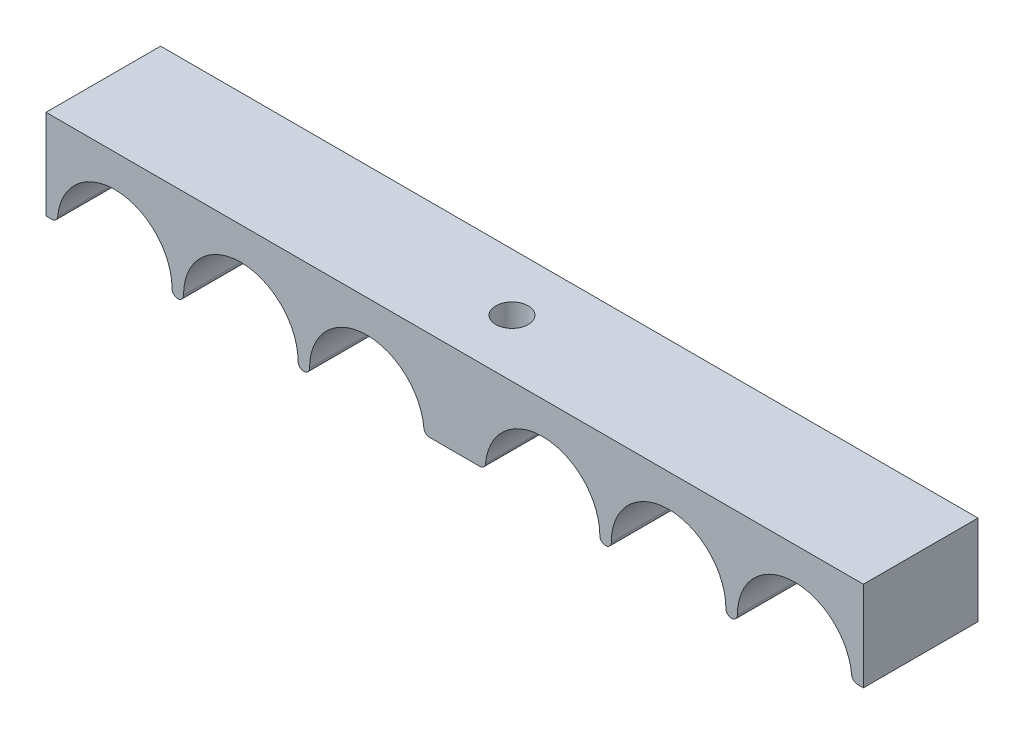
SolidWorks part; units mm, degrees
ref_plane "Front Plane" through (0, 0, 0) normal (0, 0, 1) x (1, 0, 0)
ref_plane "Top Plane" through (0, 0, 0) normal (0, 1, 0) x (1, 0, 0)
ref_plane "Right Plane" through (0, 0, 0) normal (1, 0, 0) x (0, 0, -1)
sketch "Sketch1" plane through (0, 0, 0) normal (0, 0, 1) x (1, 0, 0)
  line L0 (-107, 0) -> (-107, 23.5)
  line L1 (-107, 23.5) -> (107, 23.5)
  line L2 (107, 0) -> (-107, 0) construction
  line L3 (-89, 47.3416) -> (-89, -26.6733) construction
  line L4 (-107, 0) -> (-105.4317, 0)
  line L5 (-56, 0) -> (-56, -36.4967) construction
  line L6 (-23, 0) -> (-23, -38.0165) construction
  line L7 (6.5683, 0) -> (-6.5683, 0)
  line L8 (0, 0) -> (0, 56.3433) construction
  line L9 (107, 0) -> (105.4317, 0)
  line L10 (107, 0) -> (107, 23.5)
  arc A0 (-74, 0) -> (-103.9379, 1.3636) centre (-89, 0) ccw
  arc A1 (-41, 0) -> (-71, 0) centre (-56, 0) ccw
  arc A2 (-8.0621, 1.3636) -> (-38, 0) centre (-23, 0) ccw
  arc A3 (-105.4317, 0) -> (-103.9379, 1.3636) centre (-105.4317, 1.5) ccw
  arc A4 (-74, 0) -> (-71, 0) centre (-72.5, 0) ccw
  arc A5 (-41, 0) -> (-38, 0) centre (-39.5, 0) ccw
  arc A6 (-8.0621, 1.3636) -> (-6.5683, 0) centre (-6.5683, 1.5) ccw
  arc A7 (8.0621, 1.3636) -> (6.5683, 0) centre (6.5683, 1.5) cw
  arc A8 (41, 0) -> (38, 0) centre (39.5, 0) cw
  arc A9 (74, 0) -> (71, 0) centre (72.5, 0) cw
  arc A10 (105.4317, 0) -> (103.9379, 1.3636) centre (105.4317, 1.5) cw
  arc A11 (8.0621, 1.3636) -> (38, 0) centre (23, 0) cw
  arc A12 (41, 0) -> (71, 0) centre (56, 0) cw
  arc A13 (74, 0) -> (103.9379, 1.3636) centre (89, 0) cw
  point P42 (0, 23.5)
  dimension "D4" = 30
  dimension "D8" = 1.5
  dimension "D7" = 1.5
  dimension "D1" = 107
  dimension "D2" = 23.5
  dimension "D3" = 18
  dimension "D6" = 33
  dimension "D5" = 3
extrude "Boss-Extrude1" add sketch "Sketch1" along normal blind 30
hole_wizard "M10 Tapped Hole1" positions "Sketch3" profile "Sketch4" tap size "M10" standard "GB" end condition through all
sketch "Sketch3" plane through (0, 23.5, 0) normal (0, 1, 0) x (-1, 0, 0)
  line L0 (-107, 0) -> (107, 0) construction
  line L1 (107, 30) -> (107, 0) construction
  point P0 (0, 15)
  dimension "D1" = 15
  dimension "D2" = 107
sketch "Sketch4" plane through (0, 23.5, 15) normal (1, 0, 0) x (0, 0, 1)
  line L0 (0, 0) -> (0, 25)
  line L1 (0, 25) -> (4.25, 25)
  line L2 (4.25, 25) -> (4.25, 0)
  line L5 (4.25, 0) -> (0, 0)
  line L11 (0, -6.35) -> (0, 107.95) construction
  dimension "通孔螺纹孔钻头直径" = 8.5
  dimension "通孔螺纹孔钻头深度" = 25
cosmetic thread "Cosmetic Thread1" parameters "D2"=10
